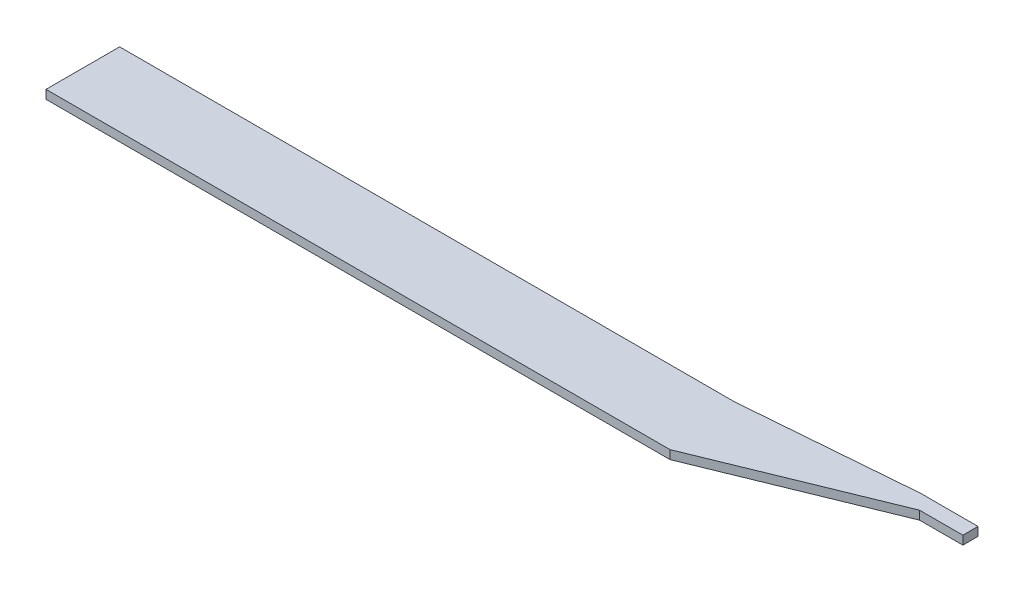
from build123d import *

# Parameters (mm, degrees)
BOSS_EXTRUDE1_DEPTH = 0.2


with BuildPart() as part:
    # Sketch1 → Boss-Extrude1 (new body)
    with BuildSketch(Plane(origin=(0, 0, 0), x_dir=(1, 0, 0), z_dir=(0, 1, 0))):
        Polygon((19.5, 1.67), (18.5, 1.67), (14.40778992, 0), (0, 0), (0, 1.7), (14.2, 1.7), (18.177225926, 2.02), (19.5, 2.02), align=None)
    extrude(amount=BOSS_EXTRUDE1_DEPTH)


solid = part.part
